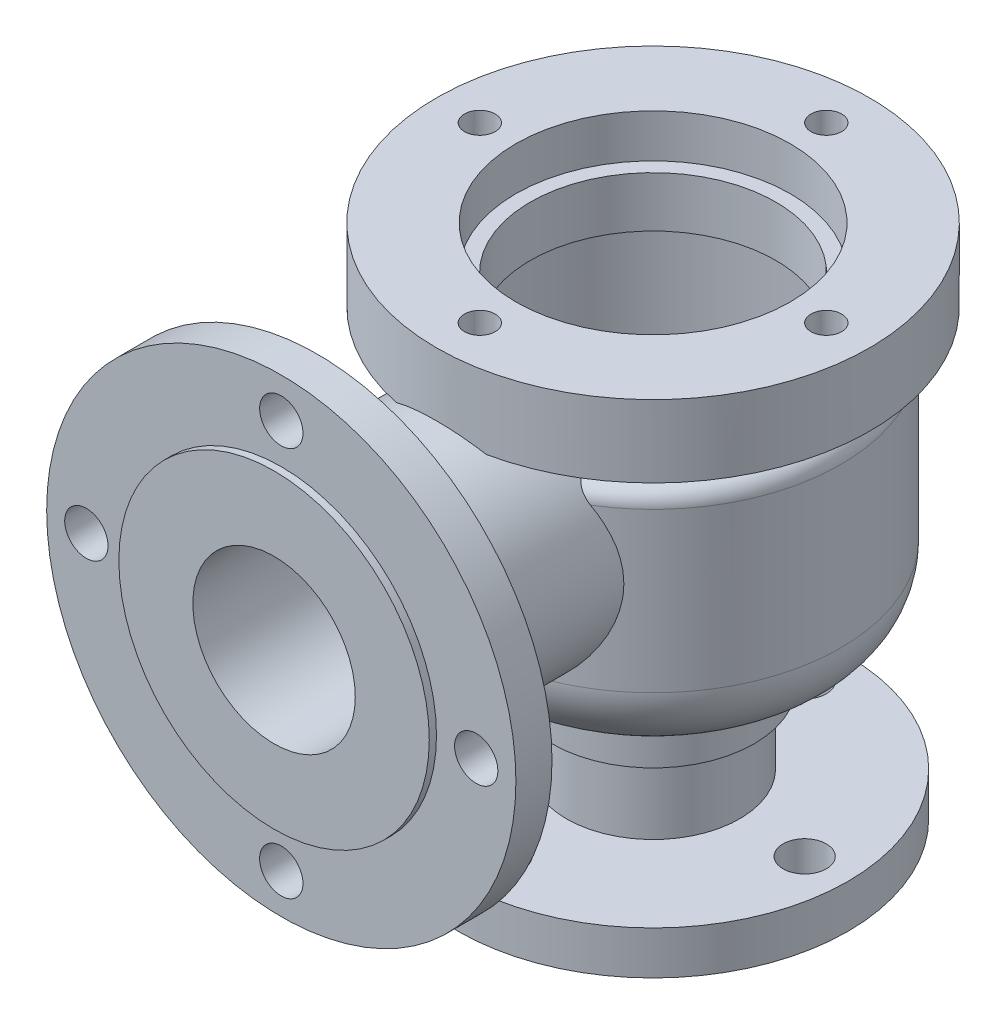
from build123d import *

# Parameters (mm, degrees)
CUT_EXTRUDE1_DEPTH         = 120
CUT_EXTRUDE2_REACH         = 239.474
SKETCH5_R                  = 6
CUT_EXTRUDE3_REACH         = 202.534
SKETCH6_R                  = 6
M10_TAPPED_HOLE1_D         = 8.5
M10_TAPPED_HOLE1_DEPTH     = 24.5
M10_TAPPED_HOLE1_TIP       = 2.553657631
SKETCH11_W                 = 2.5
SKETCH11_H                 = 60
M6_TAPPED_HOLE1_AT_2_COUNT = 2
M6_TAPPED_HOLE1_AT_2_PITCH = 30


with BuildPart() as part:
    # Sketch1 → Revolve1 (revolve)
    with BuildSketch(Plane(origin=(0, 0, 0), x_dir=(0, 0, -1), z_dir=(1, 0, 0)), mode=Mode.PRIVATE) as revolve1_sk:
        with BuildLine():
            Line((0, 0), (32, 0))
            Line((32, 0), (32, 2))
            Line((32, 2), (54, 2))
            Line((54, 2), (54, 14))
            Line((54, 14), (24, 14))
            Line((24, 14), (24, 34))
            Line((24, 34), (28, 34))
            Line((28, 34), (28, 46))
            ThreePointArc((28, 46), (28.878679656, 48.121320344), (31, 49))
            Line((31, 49), (32, 49))
            ThreePointArc((32, 49), (46.142135624, 54.857864376), (52, 69))
            Line((52, 69), (52, 113))
            ThreePointArc((52, 113), (50.535533906, 116.535533906), (47, 118))
            ThreePointArc((47, 118), (44.878679656, 118.878679656), (44, 121))
            ThreePointArc((44, 121), (45.171572875, 123.828427125), (48, 125))
            Line((48, 125), (60, 125))
            Line((60, 125), (60, 145))
            Line((60, 145), (0, 145))
            Line((0, 145), (0, 0))
        make_face()
    revolve(revolve1_sk.sketch.rotate(Axis((0, 101.241041823, 0), (0, -1, 0)), 180), axis=Axis((0, 101.241041823, 0), (0, -1, 0)))

    # Sketch2 → Revolve2 (revolve)
    with BuildSketch(Plane(origin=(0, 0, 0), x_dir=(0, 0, -1), z_dir=(1, 0, 0)), mode=Mode.PRIVATE) as revolve2_sk:
        Polygon((-105, 117.5), (-105, 138), (-103, 138), (-103, 160), (-93, 160), (-93, 127.5), (-37.396754558, 127.5), (-37.396754558, 95), (-41.57405161, 95), (-41.57405161, 117.5), align=None)
    revolve(revolve2_sk.sketch.rotate(Axis((0, 95, 163.31242283), (0, 0, -1)), 90), axis=Axis((0, 95, 163.31242283), (0, 0, -1)))

    # Sketch3 → Cut-Extrude1 (cut)
    with BuildSketch(Plane.XY.offset(105)):
        with BuildLine():
            ThreePointArc((15.81929202, 111), (0, 117.5), (-15.81929202, 111))
            Line((-15.81929202, 111), (15.81929202, 111))
        make_face()
    extrude(amount=-CUT_EXTRUDE1_DEPTH, mode=Mode.SUBTRACT)

    # Sketch4 → Cut-Revolve1 (revolve, cut)
    with BuildSketch(Plane(origin=(0, 0, 0), x_dir=(0, 0, -1), z_dir=(1, 0, 0)), mode=Mode.PRIVATE) as cut_revolve1_sk:
        with BuildLine():
            Line((0, 145), (38, 145))
            Line((38, 145), (38, 133))
            Line((38, 133), (34, 133))
            Line((34, 133), (34, 119))
            Line((34, 119), (38.85, 119))
            Line((38.85, 119), (46, 113.000437637))
            Line((46, 113.000437637), (46, 69))
            ThreePointArc((46, 69), (41.899494937, 59.100505063), (32, 55))
            Line((32, 55), (26, 55))
            Line((26, 55), (26, 63))
            Line((26, 63), (22, 63))
            Line((22, 63), (22, 45))
            Line((22, 45), (18, 45))
            Line((18, 45), (18, 0))
            Line((18, 0), (0, 0))
            Line((0, 0), (0, 145))
        make_face()
    revolve(cut_revolve1_sk.sketch.rotate(Axis((0, 158.348136638, 0), (0, -1, 0)), 180), axis=Axis((0, 158.348136638, 0), (0, -1, 0)), mode=Mode.SUBTRACT)

    # Sketch5 → Cut-Extrude2 (cut, up to next)
    with BuildSketch(Plane.XY.offset(103), mode=Mode.PRIVATE) as cut_extrude2_sk1:
        with Locations((0, 149)):
            Circle(SKETCH5_R)
    cut_extrude2_tool1 = extrude(cut_extrude2_sk1.sketch, amount=-CUT_EXTRUDE2_REACH, mode=Mode.PRIVATE) & part.part
    # Sketch5 → Cut-Extrude2 (cut, up to next)
    with BuildSketch(Plane.XY.offset(103), mode=Mode.PRIVATE) as cut_extrude2_sk2:
        with Locations((54, 95)):
            Circle(SKETCH5_R)
    cut_extrude2_tool2 = extrude(cut_extrude2_sk2.sketch, amount=-CUT_EXTRUDE2_REACH, mode=Mode.PRIVATE) & part.part
    # Sketch5 → Cut-Extrude2 (cut, up to next)
    with BuildSketch(Plane.XY.offset(103), mode=Mode.PRIVATE) as cut_extrude2_sk3:
        with Locations((0, 41)):
            Circle(SKETCH5_R)
    cut_extrude2_tool3 = extrude(cut_extrude2_sk3.sketch, amount=-CUT_EXTRUDE2_REACH, mode=Mode.PRIVATE) & part.part
    # Sketch5 → Cut-Extrude2 (cut, up to next)
    with BuildSketch(Plane.XY.offset(103), mode=Mode.PRIVATE) as cut_extrude2_sk4:
        with Locations((-54, 95)):
            Circle(SKETCH5_R)
    cut_extrude2_tool4 = extrude(cut_extrude2_sk4.sketch, amount=-CUT_EXTRUDE2_REACH, mode=Mode.PRIVATE) & part.part
    add(cut_extrude2_tool1.solids().sort_by_distance((0, 149, 103))[0], mode=Mode.SUBTRACT)
    add(cut_extrude2_tool2.solids().sort_by_distance((54, 95, 103))[0], mode=Mode.SUBTRACT)
    add(cut_extrude2_tool3.solids().sort_by_distance((0, 41, 103))[0], mode=Mode.SUBTRACT)
    add(cut_extrude2_tool4.solids().sort_by_distance((-54, 95, 103))[0], mode=Mode.SUBTRACT)

    # Sketch6 → Cut-Extrude3 (cut, up to next)
    with BuildSketch(Plane.XZ.offset(-2), mode=Mode.PRIVATE) as cut_extrude3_sk1:
        with Locations(Location((42, 0, 0), (0, 0, 270))):
            Circle(SKETCH6_R)
    cut_extrude3_tool1 = extrude(cut_extrude3_sk1.sketch, amount=-CUT_EXTRUDE3_REACH, mode=Mode.PRIVATE) & part.part
    # Sketch6 → Cut-Extrude3 (cut, up to next)
    with BuildSketch(Plane.XZ.offset(-2), mode=Mode.PRIVATE) as cut_extrude3_sk2:
        with Locations(Location((0, -42, 0), (0, 0, 270))):
            Circle(SKETCH6_R)
    cut_extrude3_tool2 = extrude(cut_extrude3_sk2.sketch, amount=-CUT_EXTRUDE3_REACH, mode=Mode.PRIVATE) & part.part
    # Sketch6 → Cut-Extrude3 (cut, up to next)
    with BuildSketch(Plane.XZ.offset(-2), mode=Mode.PRIVATE) as cut_extrude3_sk3:
        with Locations(Location((-42, 0, 0), (0, 0, 270))):
            Circle(SKETCH6_R)
    cut_extrude3_tool3 = extrude(cut_extrude3_sk3.sketch, amount=-CUT_EXTRUDE3_REACH, mode=Mode.PRIVATE) & part.part
    # Sketch6 → Cut-Extrude3 (cut, up to next)
    with BuildSketch(Plane.XZ.offset(-2), mode=Mode.PRIVATE) as cut_extrude3_sk4:
        with Locations(Location((0, 42, 0), (0, 0, 270))):
            Circle(SKETCH6_R)
    cut_extrude3_tool4 = extrude(cut_extrude3_sk4.sketch, amount=-CUT_EXTRUDE3_REACH, mode=Mode.PRIVATE) & part.part
    add(cut_extrude3_tool1.solids().sort_by_distance((42, 2, 0))[0], mode=Mode.SUBTRACT)
    add(cut_extrude3_tool2.solids().sort_by_distance((0, 2, -42))[0], mode=Mode.SUBTRACT)
    add(cut_extrude3_tool3.solids().sort_by_distance((-42, 2, 0))[0], mode=Mode.SUBTRACT)
    add(cut_extrude3_tool4.solids().sort_by_distance((0, 2, 42))[0], mode=Mode.SUBTRACT)

    # M10 Tapped Hole1
    with Locations(Plane(origin=(0, 145, 0), x_dir=(1, 0, 0), z_dir=(0, 1, 0))):
        with Locations((0, 0), (0, 48), (48, 0), (0, -48), (-48, 0)):
            Hole(M10_TAPPED_HOLE1_D / 2, depth=M10_TAPPED_HOLE1_DEPTH)
            with Locations((0, 0, -(M10_TAPPED_HOLE1_DEPTH + M10_TAPPED_HOLE1_TIP / 2))):  # 118° drill point
                Cone(0, M10_TAPPED_HOLE1_D / 2, M10_TAPPED_HOLE1_TIP, mode=Mode.SUBTRACT)

    # Sketch11 → M6 Tapped Hole1 (revolve, cut)
    with BuildSketch(Plane(origin=(0, 76, 0), x_dir=(0, -1, 0), z_dir=(1, 0, 0))):
        with Locations((1.25, 30)):
            Rectangle(SKETCH11_W, SKETCH11_H)
    m6_tapped_hole1 = revolve(axis=Axis((0, 76, 6.35), (0, 0, -1)), mode=Mode.SUBTRACT)

    # M6 Tapped Hole1 at 2: M6 Tapped Hole1 ×2
    with Locations(*[(0, i * M6_TAPPED_HOLE1_AT_2_PITCH, 0) for i in range(1, M6_TAPPED_HOLE1_AT_2_COUNT)]):
        add(m6_tapped_hole1, mode=Mode.SUBTRACT)


solid = part.part
